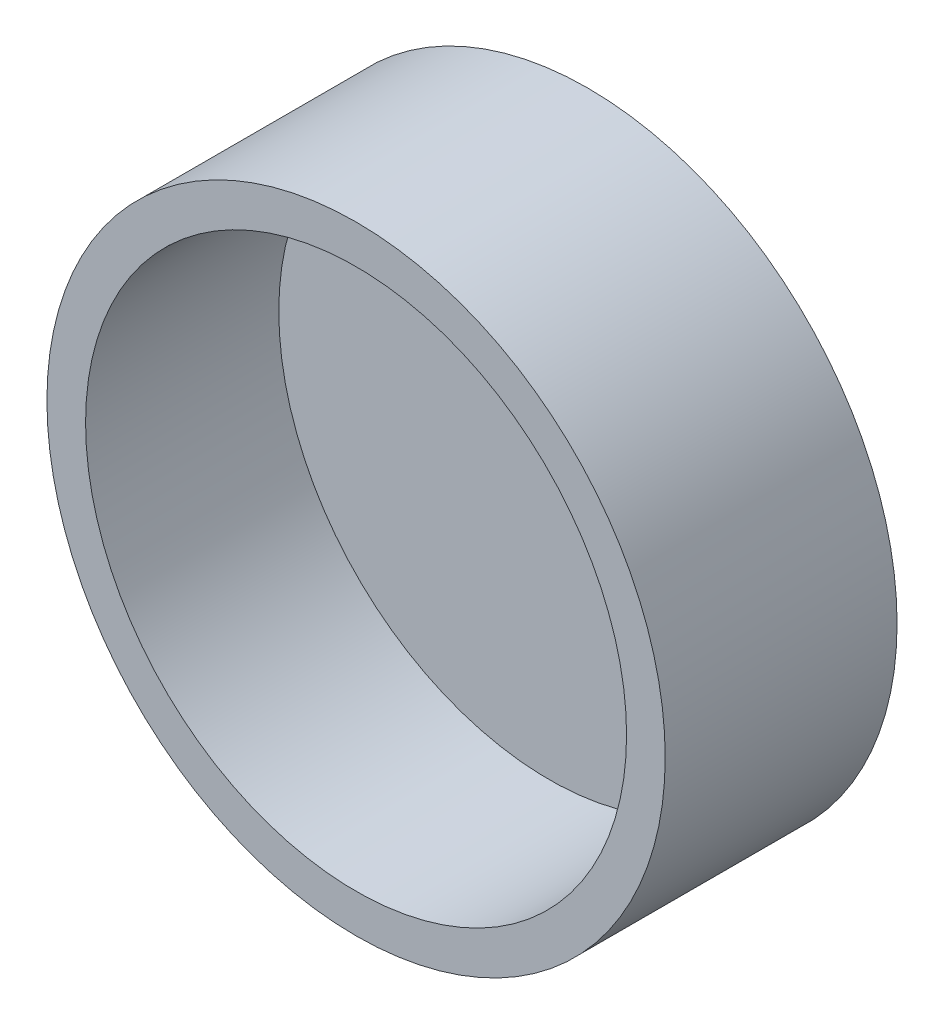
SolidWorks part; units mm, degrees
ref_plane "Front Plane" through (0, 0, 0) normal (0, 0, 1) x (1, 0, 0)
ref_plane "Top Plane" through (0, 0, 0) normal (0, 1, 0) x (1, 0, 0)
ref_plane "Right Plane" through (0, 0, 0) normal (1, 0, 0) x (0, 0, -1)
other "Configuration Table"
sketch "Sketch1" plane through (0, 0, 0) normal (0, 0, 1) x (1, 0, 0)
  circle A0 centre (0, 0) radius 40
  dimension "D1" = 80
extrude "Boss-Extrude1" add sketch "Sketch1" along normal blind 5
sketch "Sketch2" plane through (0, 0, 5) normal (0, 0, 1) x (1, 0, 0)
  circle A0 centre (0, 0) radius 40
  circle A1 centre (0, 0) radius 35
  dimension "D1" = 80
  dimension "D2" = 70
extrude "Boss-Extrude2" add sketch "Sketch2" along normal blind 25
